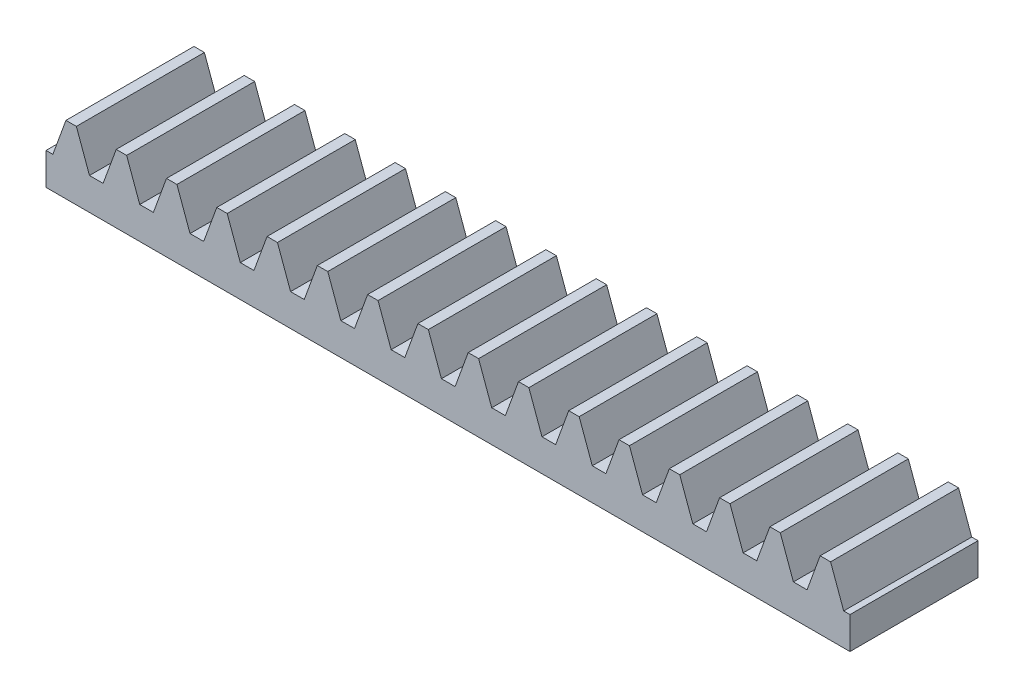
from build123d import *

# Parameters (mm, degrees)
BOSS_EXTRUDE1_DEPTH = 2
SCALE_1_SCALE       = 0.7
SKETCH2_W           = 2.409487025
SKETCH2_H           = 1.4
CUT_EXTRUDE1_DEPTH  = 10


with BuildPart() as part:
    # Sketch1 → Boss-Extrude1 (new body)
    with BuildSketch(Plane.XY):
        Polygon((7.814572092, 19.5625), (7.601354408, 19.5625), (7.396621151, 20.125), (7.233907187, 20.125), (7.02917393, 19.5625), (6.815956245, 19.5625), (6.611222988, 20.125), (6.448509024, 20.125), (6.243775767, 19.5625), (6.030558083, 19.5625), (5.825824826, 20.125), (5.663110862, 20.125), (5.458377605, 19.5625), (5.24515992, 19.5625), (5.040426663, 20.125), (4.877712699, 20.125), (4.672979442, 19.5625), (4.459761758, 19.5625), (4.255028501, 20.125), (4.092314537, 20.125), (3.88758128, 19.5625), (3.674363595, 19.5625), (3.469630338, 20.125), (3.306916374, 20.125), (3.102183117, 19.5625), (2.888965433, 19.5625), (2.684232176, 20.125), (2.521518212, 20.125), (2.316784955, 19.5625), (2.10356727, 19.5625), (1.898834013, 20.125), (1.736120049, 20.125), (1.531386792, 19.5625), (1.318169108, 19.5625), (1.113435851, 20.125), (0.950721887, 20.125), (0.74598863, 19.5625), (0.532770945, 19.5625), (0.328037688, 20.125), (0.165323724, 20.125), (-0.039409533, 19.5625), (-0.252627217, 19.5625), (-0.457360474, 20.125), (-0.620074438, 20.125), (-0.824807695, 19.5625), (-1.03802538, 19.5625), (-1.242758637, 20.125), (-1.405472601, 20.125), (-1.610205858, 19.5625), (-1.823423542, 19.5625), (-2.028156799, 20.125), (-2.190870763, 20.125), (-2.39560402, 19.5625), (-2.608821705, 19.5625), (-2.813554962, 20.125), (-2.976268926, 20.125), (-3.181002183, 19.5625), (-3.394219867, 19.5625), (-3.598953124, 20.125), (-3.761667088, 20.125), (-3.966400345, 19.5625), (-4.17961803, 19.5625), (-4.384351287, 20.125), (-4.547065251, 20.125), (-4.751798508, 19.5625), (-4.965016192, 19.5625), (-5.169749449, 20.125), (-5.332463413, 20.125), (-5.53719667, 19.5625), (-5.750414355, 19.5625), (-5.955147612, 20.125), (-6.117861576, 20.125), (-6.322594833, 19.5625), (-6.535812517, 19.5625), (-6.740545774, 20.125), (-6.903259738, 20.125), (-7.107992995, 19.5625), (-7.32121068, 19.5625), (-7.525943937, 20.125), (-7.688657901, 20.125), (-7.893391158, 19.5625), (-8, 19.5625), (-8, 19.062226191), (8, 19.062226191), (8, 20.071958989), align=None)
    extrude(amount=BOSS_EXTRUDE1_DEPTH)


with BuildPart() as part_1:
    # Scale 1: scaled about (0, 0, 0)
    add(part.part.scale(SCALE_1_SCALE))

    # Sketch2 → Cut-Extrude1 (cut)
    with BuildSketch(Plane(origin=(0, 13.343558334, 0), x_dir=(-1, 0, 0), z_dir=(0, -1, 0))):
        with Locations((-4.395256488, -0.7)):
            Rectangle(SKETCH2_W, SKETCH2_H)
    extrude(amount=-CUT_EXTRUDE1_DEPTH, mode=Mode.SUBTRACT)


solid = part_1.part
